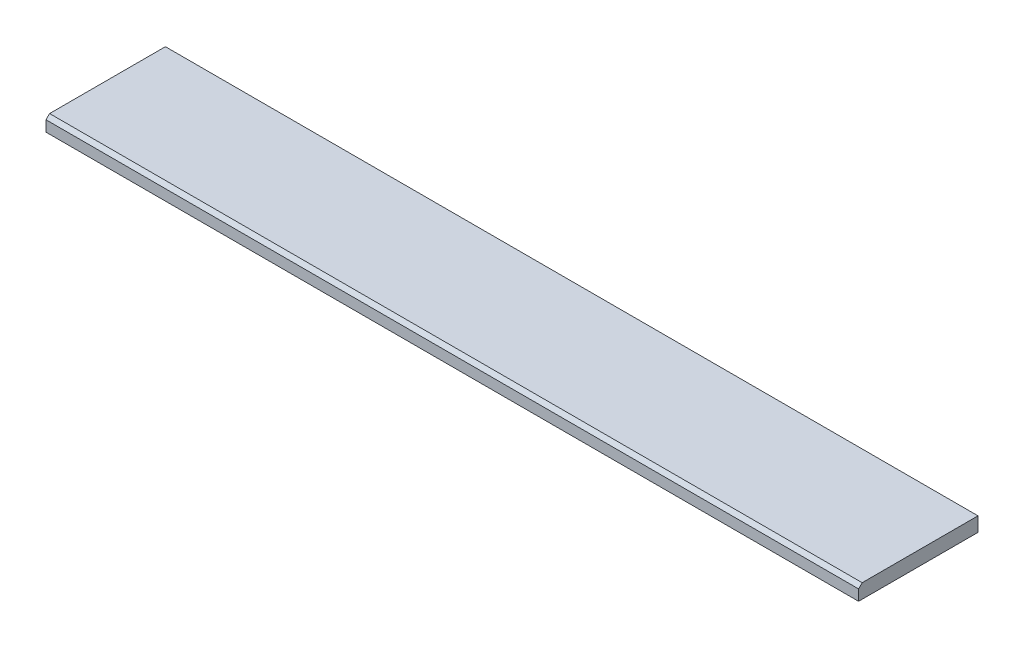
from build123d import *

# Parameters (mm, degrees)
SKETCH_1_W      = 2266
SKETCH_1_H      = 333
EXTRUDE_1_DEPTH = 40
CHAMFER_1_SIZE  = 10


with BuildPart() as part:
    # 草图1 → 凸台-拉伸1 (new body)
    with BuildSketch(Plane(origin=(0, 0, 0), x_dir=(1, 0, 0), z_dir=(0, 1, 0))):
        Rectangle(SKETCH_1_W, SKETCH_1_H)
    extrude(amount=EXTRUDE_1_DEPTH)

    # 倒角1
    chamfer_1_edges = [part.edges().sort_by_distance(p)[0] for p in [
        (0, 40, 166.5),
    ]]
    chamfer(chamfer_1_edges, length=CHAMFER_1_SIZE)


solid = part.part
